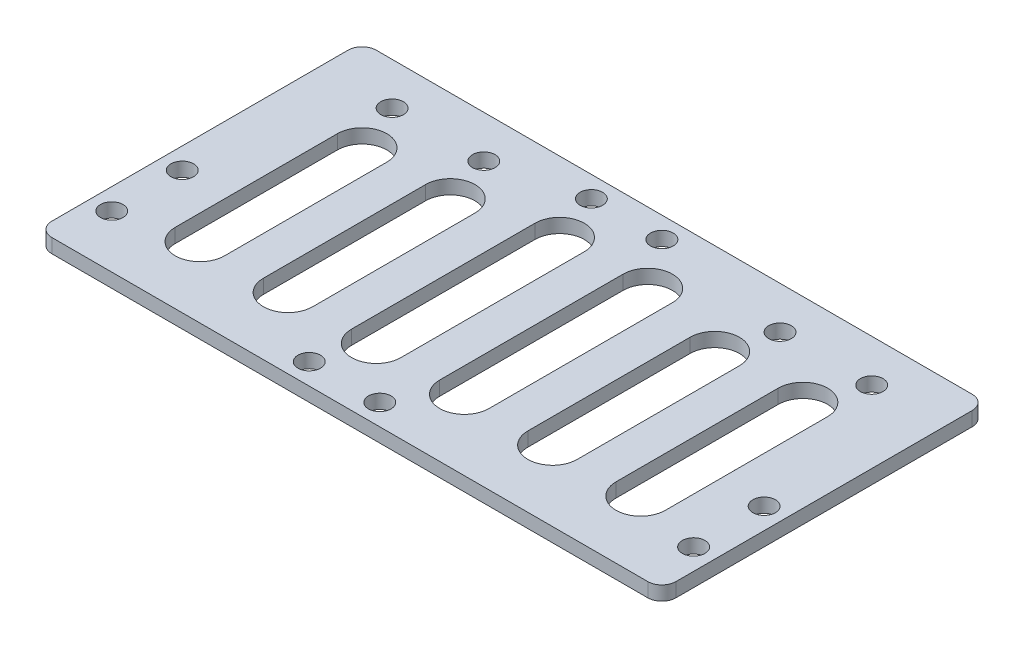
SolidWorks part; units mm, degrees
material "Thornel Mat VMA"
ref_plane "前视基准面" through (0, 0, 0) normal (0, 0, 1) x (1, 0, 0)
ref_plane "上视基准面" through (0, 0, 0) normal (0, 1, 0) x (1, 0, 0)
ref_plane "右视基准面" through (0, 0, 0) normal (1, 0, 0) x (0, 0, -1)
sketch "草图1" plane through (0, 0, 0) normal (0, 1, 0) x (1, 0, 0)
  line L0 (0, 23) -> (0, -23) construction
  line L1 (-44.25, 23) -> (44.25, 23)
  line L2 (-44.25, 23) -> (-44.25, -23)
  line L3 (-44.25, -23) -> (44.25, -23)
  line L4 (44.25, 23) -> (44.25, -23)
  line L5 (-44.25, 23) -> (44.25, -23) construction
  line L6 (-44.25, -23) -> (44.25, 23) construction
  line L7 (-41.25, -5.5) -> (-41.25, -15.5) construction
  line L8 (41.25, -5.5) -> (41.25, -15.5) construction
  line L9 (-8.75, -20) -> (1.25, -20) construction
  line L10 (-34, 17) -> (-21, 17) construction
  line L11 (21, 17) -> (34, 17) construction
  line L12 (-44.25, 0) -> (44.25, 0) construction
  line L13 (-8.75, 20) -> (1.25, 20) construction
  circle A0 centre (-41.25, -5.5) radius 1.6
  circle A1 centre (-41.25, -15.5) radius 1.6
  circle A4 centre (41.25, -15.5) radius 1.6
  circle A5 centre (41.25, -5.5) radius 1.6
  circle A6 centre (-8.75, -20) radius 1.6
  circle A7 centre (1.25, -20) radius 1.6
  circle A8 centre (-34, 17) radius 1.6
  circle A9 centre (-21, 17) radius 1.6
  circle A10 centre (21, 17) radius 1.6
  circle A11 centre (34, 17) radius 1.6
  circle A12 centre (1.25, 20) radius 1.6
  circle A13 centre (-8.75, 20) radius 1.6
  point P0 (0, 0)
  dimension "D1" = 3.2
  dimension "D7" = 3
  dimension "D9" = 13
  dimension "D11" = 3.2
  dimension "D2" = 3
  dimension "D3" = 7.5
  dimension "D4" = 10
  dimension "D5" = 46
  dimension "D6" = 88.5
  dimension "D8" = 35.5
  dimension "D10" = 6
  dimension "D12" = 42
extrude "凸台-拉伸1" add sketch "草图1" along normal blind 2
sketch "草图2" plane through (0, 2, 0) normal (0, 1, 0) x (1, 0, 0)
  line L0 (0, 23) -> (0, -23) construction
  line L1 (44.25, 23) -> (-44.25, 23) construction
  line L2 (-44.25, -23) -> (44.25, -23) construction
  line L3 (-44.25, -1.5) -> (44.25, -1.5) construction
  line L6 (-31.25, 10) -> (-31.25, -13) construction
  line L7 (-27.75, 10) -> (-27.75, -13)
  line L8 (-34.75, 10) -> (-34.75, -13)
  line L9 (-18.75, 10) -> (-18.75, -13) construction
  line L10 (-15.25, 10) -> (-15.25, -13)
  line L11 (-22.25, 10) -> (-22.25, -13)
  line L12 (-6.25, 13) -> (-6.25, -13) construction
  line L13 (-2.75, 13) -> (-2.75, -13)
  line L14 (-9.75, 13) -> (-9.75, -13)
  line L15 (6.25, 13) -> (6.25, -13) construction
  line L16 (9.75, 13) -> (9.75, -13)
  line L17 (2.75, 13) -> (2.75, -13)
  line L18 (18.75, 10) -> (18.75, -13) construction
  line L19 (22.25, 10) -> (22.25, -13)
  line L20 (15.25, 10) -> (15.25, -13)
  line L21 (31.25, 10) -> (31.25, -13) construction
  line L22 (34.75, 10) -> (34.75, -13)
  line L23 (27.75, 10) -> (27.75, -13)
  line L24 (44.25, -23) -> (44.25, 23) construction
  line L27 (-44.25, 23) -> (-44.25, -23) construction
  arc A0 (-27.75, 10) -> (-34.75, 10) centre (-31.25, 10) ccw
  arc A1 (-34.75, -13) -> (-27.75, -13) centre (-31.25, -13) ccw
  arc A2 (-15.25, 10) -> (-22.25, 10) centre (-18.75, 10) ccw
  arc A3 (-22.25, -13) -> (-15.25, -13) centre (-18.75, -13) ccw
  arc A4 (-2.75, 13) -> (-9.75, 13) centre (-6.25, 13) ccw
  arc A5 (-9.75, -13) -> (-2.75, -13) centre (-6.25, -13) ccw
  arc A6 (9.75, 13) -> (2.75, 13) centre (6.25, 13) ccw
  arc A7 (2.75, -13) -> (9.75, -13) centre (6.25, -13) ccw
  arc A8 (22.25, 10) -> (15.25, 10) centre (18.75, 10) ccw
  arc A9 (15.25, -13) -> (22.25, -13) centre (18.75, -13) ccw
  arc A10 (34.75, 10) -> (27.75, 10) centre (31.25, 10) ccw
  arc A11 (27.75, -13) -> (34.75, -13) centre (31.25, -13) ccw
  circle A14 centre (-8.75, -20) radius 1.6 construction
  circle A15 centre (-8.75, 20) radius 1.6 construction
  point P14 (-31.25, -1.5)
  point P22 (-18.75, -1.5)
  point P29 (-6.25, 0)
  point P36 (6.25, 0)
  point P43 (18.75, -1.5)
  point P50 (31.25, -1.5)
  dimension "D1" = 3.5
  dimension "D2" = 23
  dimension "D4" = 12.5
  dimension "D5" = 7
  dimension "D3" = 7
extrude "切除-拉伸1" cut sketch "草图2" against normal through all
fillet "圆角1" radius 2 4 edges at (44.25, 1, -23) (44.25, 1, 23) (-44.25, 1, 23) (-44.25, 1, -23)
